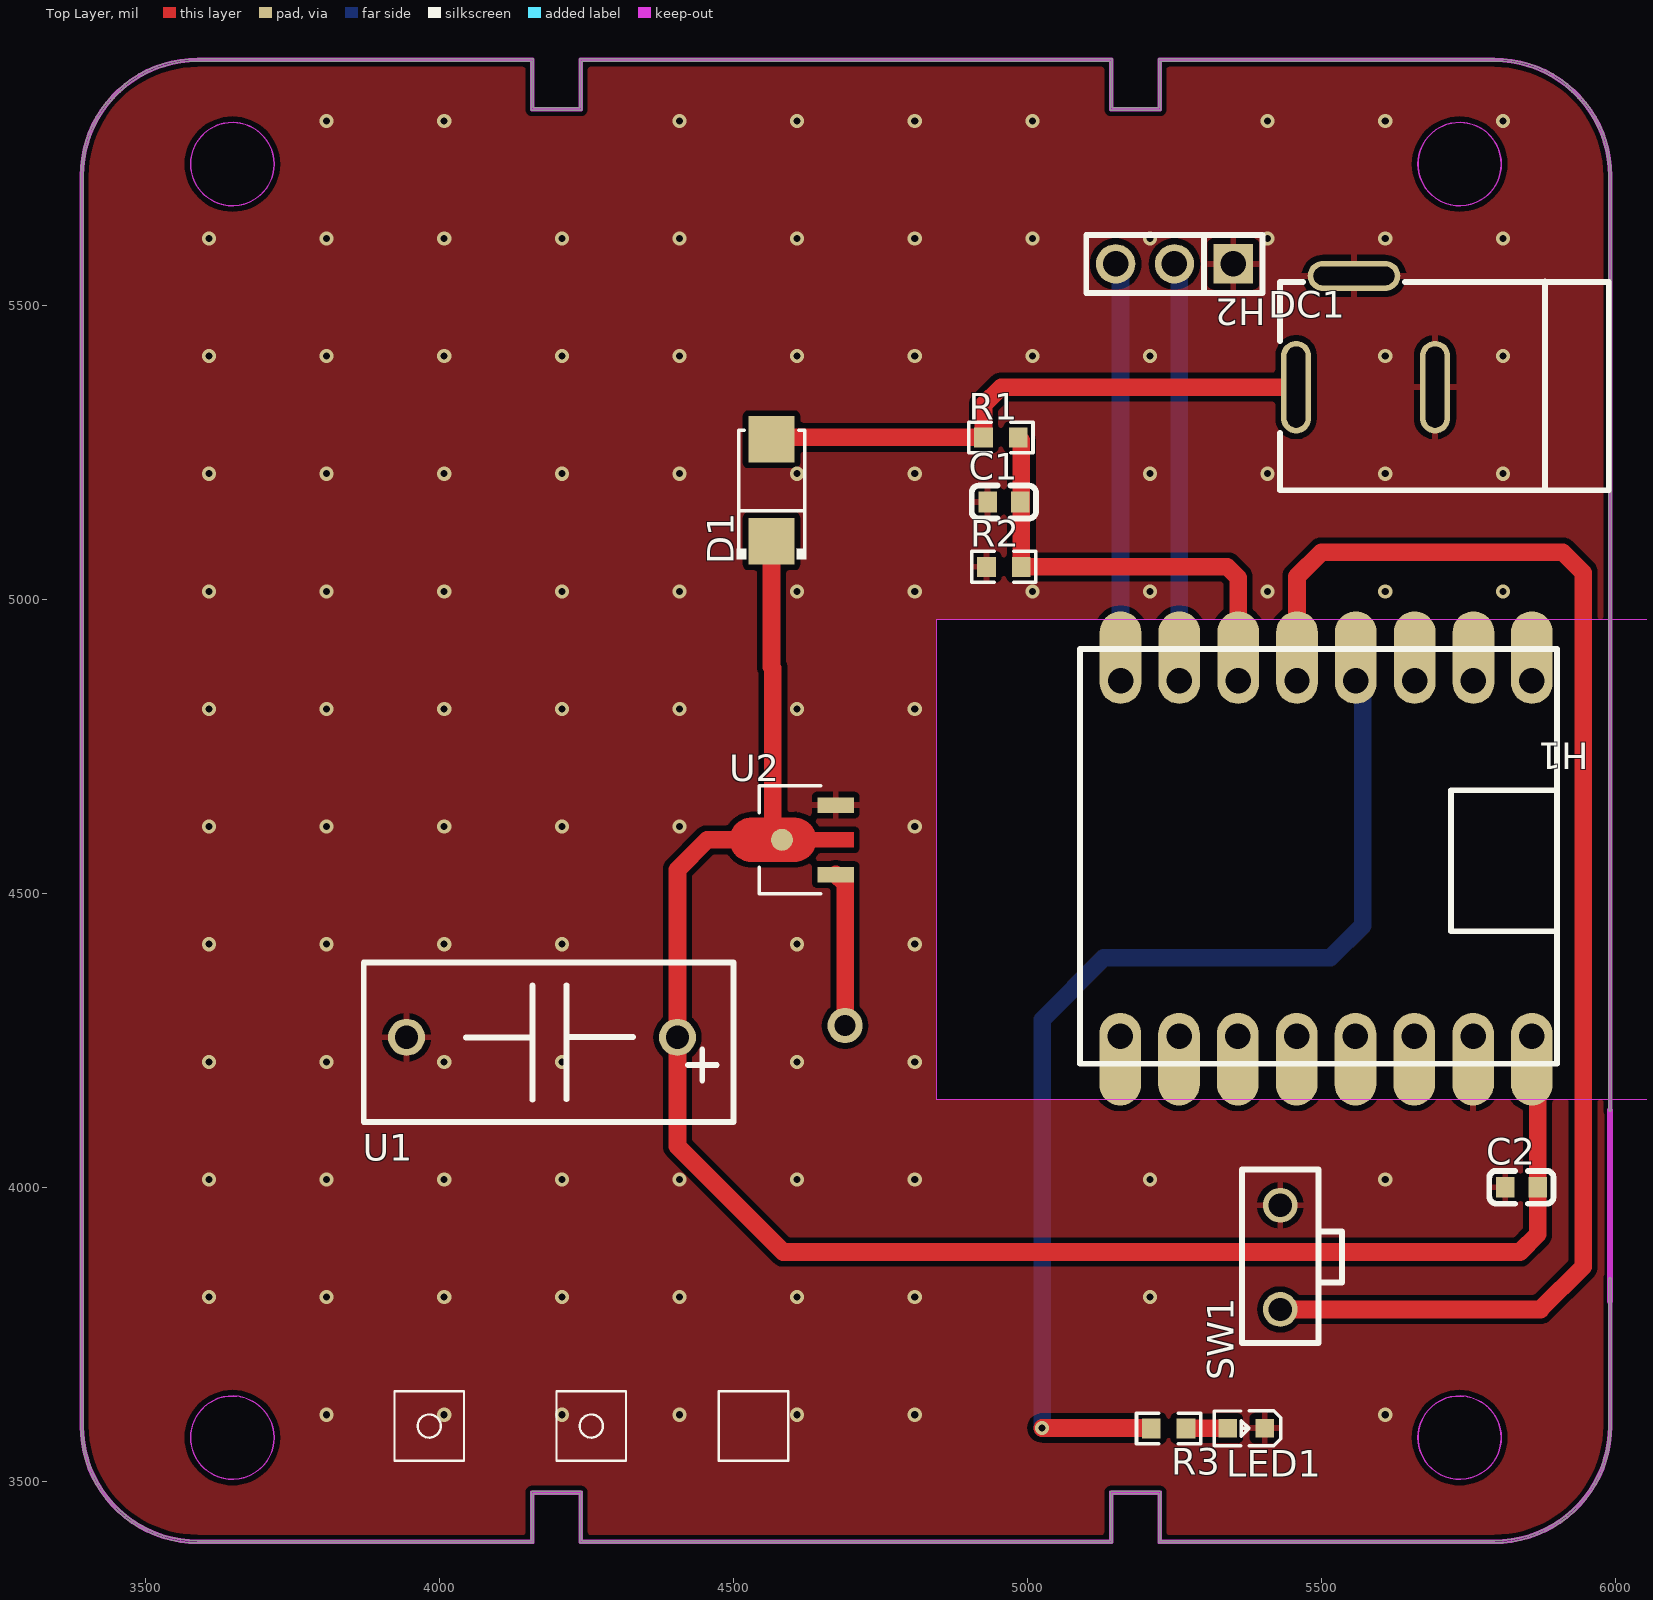
[diagram p0: Top Layer view]
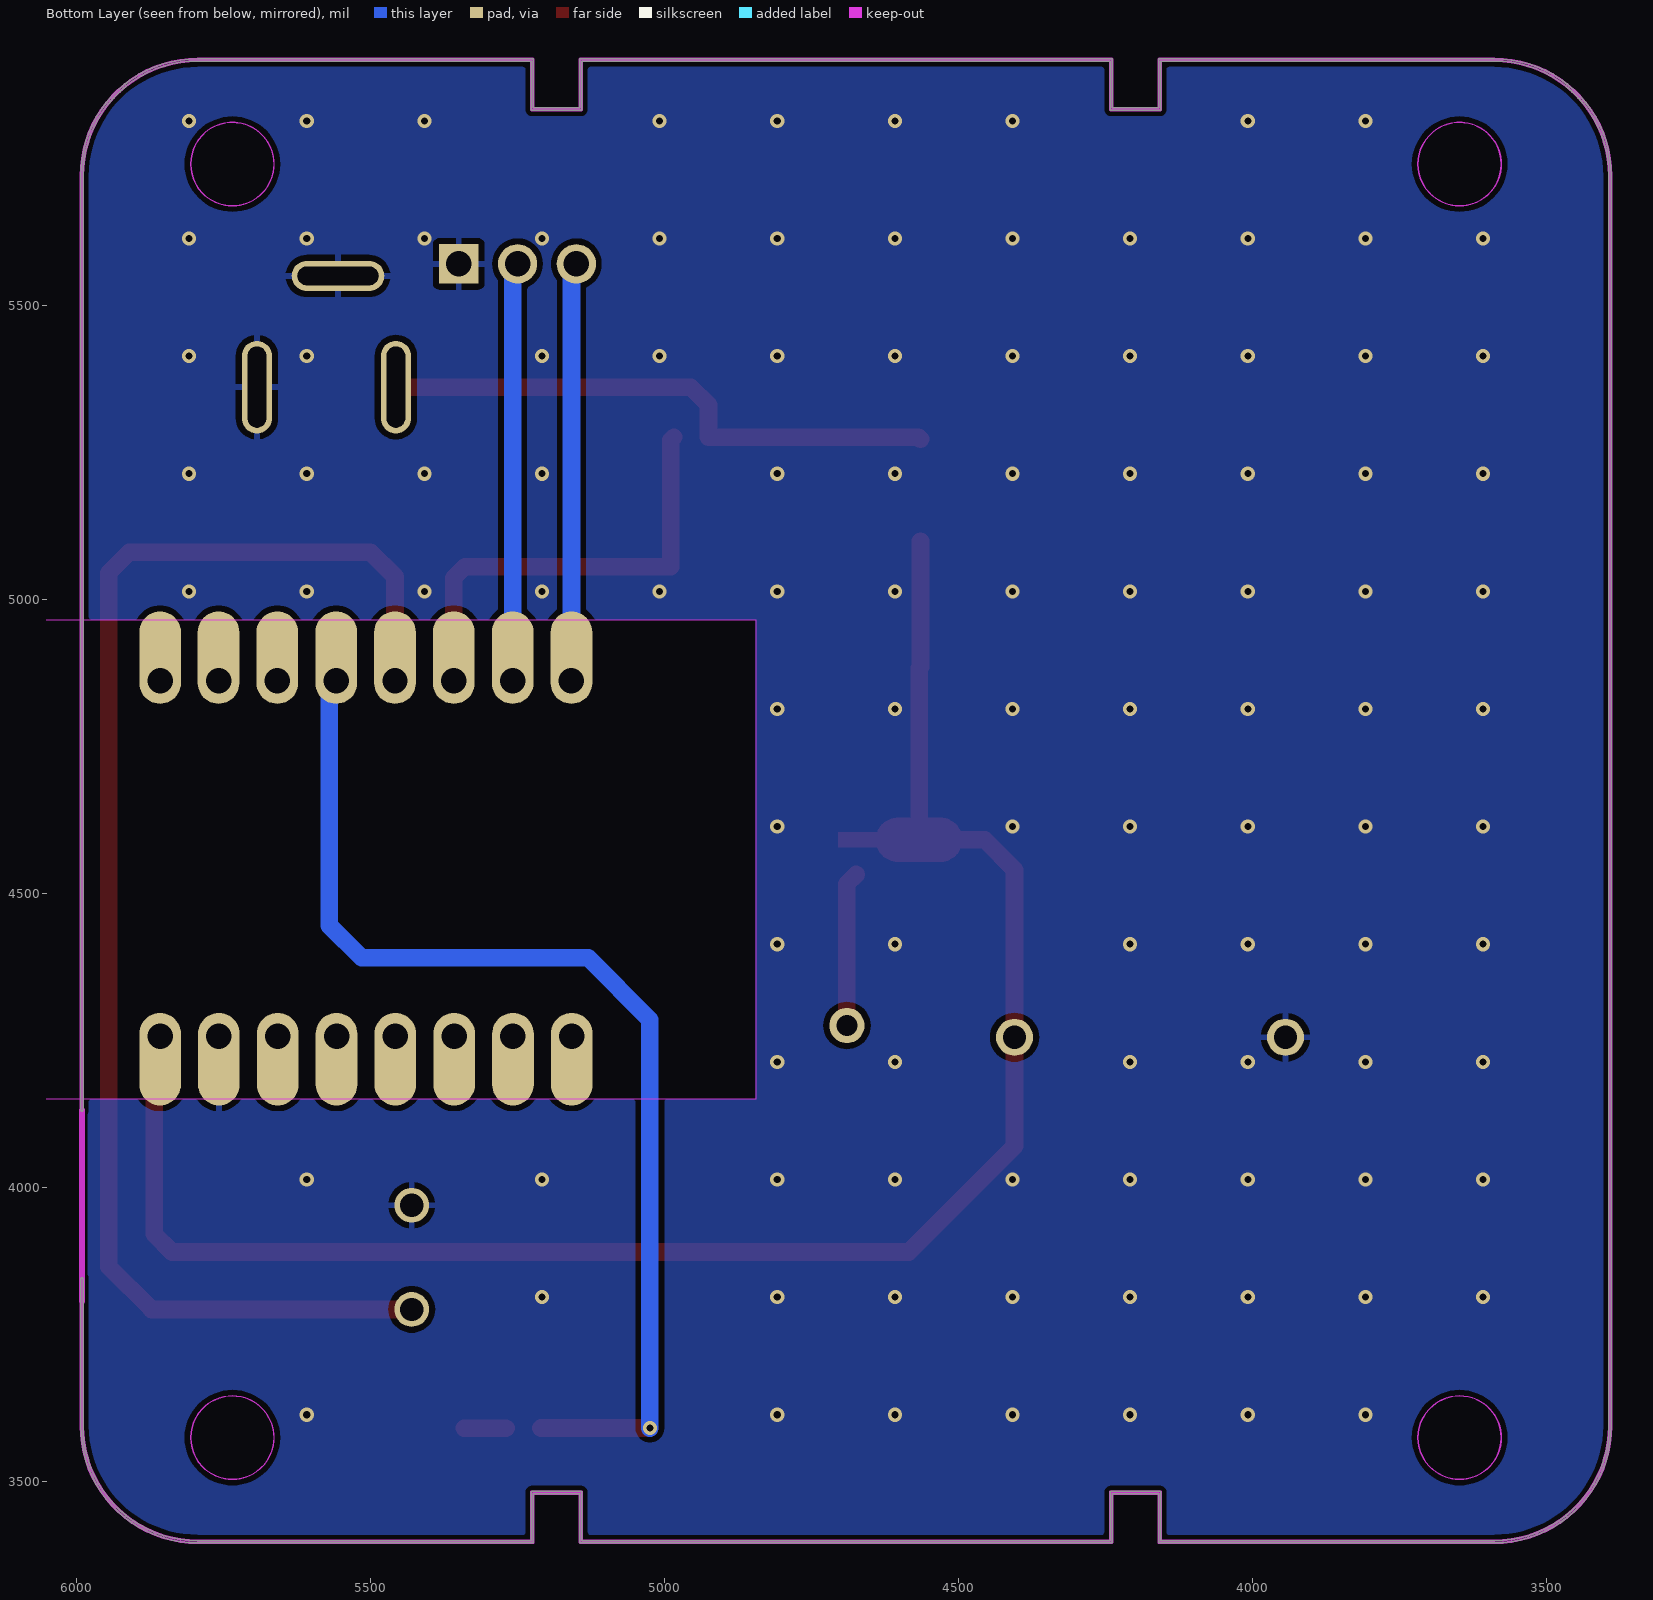
[diagram p1: Bottom Layer view, seen from below]
# Altium PCB MISC52083.pcbdoc
Units mil, origin at the board's own origin, x right, y up, seen from the top; angles counter-clockwise.
Board outline 2602.36 x 2523.62 mil, 2 copper layers (Top Layer, Bottom Layer), stack 62.206 mil thick; 13 components, 10 nets, 44 pads, 105 vias.

## Layer stack, top to bottom
Top Solder Mask Layer: solder mask 0.394, Dk 3.3
Top Layer: signal copper 1.379
Dielectric1: surface 59.449, FR4, Dk 4.5
Bottom Layer: signal copper 1.378
Bottom Solder Mask Layer: solder mask 0.394, Dk 3.3

## Board outline
5992.74,3594.03 cw(c5793.92,3594.03) 5793.92,3395.21 5224.89,3395.21 cw(c5224.89,3397.18) 5222.92,3397.18 5222.92,3478.94 5144.46,3478.94 5144.46,3397.18 cw(c5142.49,3397.18) 5142.49,3395.21 4240.63,3395.21 cw(c4240.63,3397.18) 4238.67,3397.18 4238.67,3478.94 4160.21,3478.94 4160.21,3397.18 cw(c4158.24,3397.18) 4158.24,3395.21 3589.2,3395.21 cw(c3589.2,3594.03) 3390.38,3594.03 3390.38,5720.02 cw(c3589.2,5720.02) 3589.2,5918.84 4158.24,5918.84 cw(c4158.24,5916.87) 4160.21,5916.87 4160.21,5835.12 4238.67,5835.12 4238.67,5916.87 cw(c4240.63,5916.87) 4240.63,5918.84 5142.49,5918.84 cw(c5142.49,5916.87) 5144.46,5916.87 5144.46,5835.12 5222.92,5835.12 5222.92,5916.87 cw(c5224.89,5916.87) 5224.89,5918.84 5793.92,5918.84 cw(c5793.92,5720.02) 5992.74,5720.02 5992.74,4131.27 cw(c5990.77,4131.27) 5990.77,4129.3 cw(c5990.77,4131.27) 5988.81,4131.27 5988.81,5720.02 ccw(c5793.92,5720.02) 5793.92,5914.9 5226.85,5914.9 5226.85,5833.16 cw(c5224.89,5833.16) 5224.89,5831.19 5142.49,5831.19 cw(c5142.49,5833.16) 5140.52,5833.16 5140.52,5914.9 4242.6,5914.9 4242.6,5833.16 cw(c4240.63,5833.16) 4240.63,5831.19 4158.24,5831.19 cw(c4158.24,5833.16) 4156.27,5833.16 4156.27,5914.9 3589.2,5914.9 ccw(c3589.2,5720.02) 3394.32,5720.02 3394.32,3594.03 ccw(c3589.2,3594.03) 3589.2,3399.15 4156.27,3399.15 4156.27,3480.91 cw(c4158.24,3480.91) 4158.24,3482.87 4240.63,3482.87 cw(c4240.63,3480.91) 4242.6,3480.91 4242.6,3399.15 5140.52,3399.15 5140.52,3480.91 cw(c5142.49,3480.91) 5142.49,3482.87 5224.89,3482.87 cw(c5224.89,3480.91) 5226.85,3480.91 5226.85,3399.15 5793.92,3399.15 ccw(c5793.92,3594.03) 5988.81,3594.03 5988.81,3844.2 cw(c5990.77,3844.2) 5990.77,3846.17 cw(c5990.77,3844.2) 5992.74,3844.2 5992.74,3594.03
cut-out: 3719.12,3574.35 cw(c3648.26,3574.35) 3577.39,3574.35 cw(c3648.26,3574.35)
cut-out: 5805.74,5739.7 cw(c5734.87,5739.7) 5664,5739.7 cw(c5734.87,5739.7)
cut-out: 3719.12,5739.7 cw(c3648.26,5739.7) 3577.39,5739.7 cw(c3648.26,5739.7)
cut-out: 5805.74,3574.35 cw(c5734.87,3574.35) 5664,3574.35 cw(c5734.87,3574.35)

## Design rules (kind name [scope] priority, off if disabled: settings)
BoardOutlineClearance copperThickness2oz_1 [All] p2 off: genericclearance=7.99 ignorepadtopadclearanceinfootprint=FALSE except(0: Arc-SplitContinuation Track-SplitContinuation SMDPad-SplitContinuation THPad-SplitContinuation Via-SplitContinuation Fill-SplitContinuation Region-SplitContinuation Poly-SplitContinuation Text-SplitContinuation Hole-SplitContinuation; 5.98: Arc-CutoutEdge SMDPad-CutoutEdge THPad-CutoutEdge Via-CutoutEdge Fill-CutoutEdge Region-CutoutEdge Text-CutoutEdge; 6.93: Hole-OutlineEdge Hole-CutoutEdge; 10: Poly-OutlineEdge Poly-CutoutEdge; 11.81: Arc-OutlineEdge Track-OutlineEdge SMDPad-OutlineEdge THPad-OutlineEdge Via-OutlineEdge Fill-OutlineEdge Region-OutlineEdge Text-OutlineEdge Track-CutoutEdge)
BoardOutlineClearance copperThickness1oz_1 [All] p4: genericclearance=4.02 ignorepadtopadclearanceinfootprint=FALSE except(0: Arc-SplitContinuation Track-SplitContinuation SMDPad-SplitContinuation THPad-SplitContinuation Via-SplitContinuation Fill-SplitContinuation Region-SplitContinuation Poly-SplitContinuation Text-SplitContinuation Hole-SplitContinuation; 6: SMDPad-CutoutEdge THPad-CutoutEdge Via-CutoutEdge Fill-CutoutEdge Region-CutoutEdge Text-CutoutEdge; 6.93: Hole-OutlineEdge Hole-CutoutEdge; 10: Poly-OutlineEdge Poly-CutoutEdge; 11.8: Arc-OutlineEdge Track-OutlineEdge SMDPad-OutlineEdge THPad-OutlineEdge Via-OutlineEdge Fill-OutlineEdge Region-OutlineEdge Text-OutlineEdge; 11.81: Arc-CutoutEdge Track-CutoutEdge)
Clearance copperThickness2oz [All] p1 off: gap=7.99 ignorepadtopadclearanceinfootprint=FALSE except(5.98: SMDPad-Track SMDPad-SMDPad THPad-Track SMDPad-THPad THPad-THPad Track-Via SMDPad-Via THPad-Via Via-Via Fill-Track Region-Track Fill-SMDPad Region-SMDPad Fill-THPad Region-THPad Fill-Via Region-Via Fill-Fill Fill-Region Region-Region Arc-Track Arc-SMDPad Arc-THPad Arc-Via Fill-Arc Region-Arc Arc-Arc Text-Track SMDPad-Text Text-THPad Text-Via Fill-Text Region-Text Arc-Text Text-Text; 6.93: Hole-Track Hole-SMDPad Hole-THPad Hole-Via Fill-Hole Region-Hole Hole-Arc Hole-Text; 10: Poly-Track Poly-SMDPad Poly-THPad Poly-Via Poly-Fill Poly-Region Poly-Poly Poly-Arc Poly-Text Poly-Hole)
Clearance copperThickness1oz [All] p3: gap=4.02 ignorepadtopadclearanceinfootprint=FALSE except(5.98: SMDPad-Track SMDPad-SMDPad THPad-Track SMDPad-THPad THPad-THPad Track-Via SMDPad-Via THPad-Via Via-Via Fill-Track Region-Track Fill-SMDPad Region-SMDPad Fill-THPad Region-THPad Fill-Via Region-Via Fill-Fill Fill-Region Region-Region; 6: Arc-Track Arc-SMDPad Arc-THPad Arc-Via Fill-Arc Region-Arc Arc-Arc Text-Track SMDPad-Text Text-THPad Text-Via Fill-Text Region-Text Arc-Text Text-Text; 6.93: Hole-Track Hole-SMDPad Hole-THPad Hole-Via Fill-Hole Region-Hole Hole-Arc Hole-Text; 10: Poly-Track Poly-SMDPad Poly-THPad Poly-Via Poly-Fill Poly-Region Poly-Poly Poly-Arc Poly-Text Poly-Hole)
Creepage creepage [All] p1: checkdistance=0 ignoreinternallayers=TRUE applytopolygonpour=TRUE
DiffPairsRouting differentialPair [All] p1: maxlimit=6 minlimit=6 mostfreqgap=6 toplayer_minwidth=5 toplayer_prefwidth=10 toplayer_maxwidth=100 toplayer_mingap=6 toplayer_prefgap=6 toplayer_maxgap=6 bottomlayer_minwidth=5 bottomlayer_prefwidth=10 bottomlayer_maxwidth=100 bottomlayer_mingap=6 bottomlayer_prefgap=6 bottomlayer_maxgap=6 maxuncoupledlength=10
HoleToHoleClearance otherClearance [All] p1: gap=11.81 allowstackedmicrovias=TRUE
Length netLength [All] p1: minlimit=0 maxlimit=0
MatchedLengths netLengthTolerance [All] p1: tolerance=1000
PasteMaskExpansion pasteMaskExpansion [All] p1: expansion=0
PlaneConnect innerPlane [All] p1: planeconnectstyle=Relief reliefexpansion=20 reliefentries=4 reliefconductorwidth=10 reliefairgap=10
PolygonConnect copperRegion [(InNet('GND'))] p1: connectstyle=Relief reliefconductorwidth=10 reliefentries=4 polygonreliefangle="90 Angle" airgapwidth=10 via.connectstyle=Relief via.reliefconductorwidth=10 via.reliefentries=4 via.polygonreliefangle="90 Angle" via.airgapwidth=10
RoutingVias viaSize [All] p1: holewidth=12.01 width=24.02 viastyle="Through Hole" minholewidth=11.81 minwidth=19.68 maxholewidth=248.03 maxwidth=393.7
SolderMaskExpansion solderMaskExpansion [IsVia] p1: expansion=-1000 istentingtop=TRUE
SolderMaskExpansion solderMaskExpansion [All] p2: expansion=2 istentingtop=FALSE
Width copperThickness2oz_2 [All] p1 off: maxlimit=100 minlimit=8 preferedwidth=10
Width copperThickness1oz_2 [All] p2: maxlimit=100 minlimit=5 preferedwidth=10

## Components (designator, comment, footprint, x,y, rotation, side; value= is the part's Value field where it differs from the comment)
C1 "100nF" C0603 4960,5165 r0 top
C2 "100nF" C0603 5840,4000 r0 top
D1 "SS34" SMA_L4.3-W2.6-LS5.2-RD 4565,5185 r90 top
DC1 "" DC-2.0 5580,5350 r0 top
H1 "" HDR-TH_16P-P2.54-V-F-R2-C8-S2.54-1 5545,4865 r180 top
H2 "" HDR-TH_3P-P2.54-V-M 5250,5570 r180 top
LED1 "" LED_0603 5370,3590 r180 top
R1 "10K" R0603 4955,5275 r180 top
R2 "15K" R0603 4960,5055 r0 top
R3 "1K" R0603 5240,3590 r0 top
SW1 "" Key_TH_3.5x6x4.3 5430,3835 r90 top
U1 "2F" CAP-TH_BD8.0-P3.50-D0.6-FD_GDC02R7R205LD0816 4405,4255 r180 top
U2 "HT7033A-1" SOT-89-3_L4.5-W2.5-P1.50-LS4.2-BR 4620.69,4590.78 r0 top

## Footprints (in the part's own frame and the unit in brackets; to place one, negate y for a bottom-side part, rotate by r counter-clockwise, add the part's x,y. Pads: shape width x height; smd on the part's side, far side on the other; paste and mask are expansions set on the pad)
C0603 [mm]
  rect 0.8x0.9 smd: 1(-0.7,0) 2(0.7,0)
  silkscreen extent -1.39,-0.71 1.39,0.71
CAP-TH_BD8.0-P3.50-D0.6-FD_GDC02R7R205LD0816 [mm]
  round 1.6 hole 1: 1(0,0) 2(11.7,0)
  silkscreen extent -2.42,-3.22 13.55,3.65
DC-2.0 [mil]
  oval 157.5x51.2 hole 31.5 slot 137.8 at 0 deg paste+0 mask+2: 2(-24.7,199.5)
  oval 51.2x157.5 hole 31.5 slot 137.8 at 90 deg paste+0 mask+2: 3(113.1,10.5) 4(-123.1,10.5)
  silkscreen extent -151,-165 408,190
HDR-TH_3P-P2.54-V-M [mm]
  rect 1.7x1.7 hole 1.1: 1(-2.54,0)
  round 1.7 hole 1.1: 2(0,0) 3(2.54,0)
  silkscreen extent -3.81,-1.25 3.81,1.25
HDR-TH_16P-P2.54-V-F-R2-C8-S2.54-1 [mm]
  oval 1.8x4 hole 1.1 copper offset 0,1: 1(-7.945,15.439) 3(-5.405,15.439) 5(-2.865,15.439) 7(-0.325,15.439) 9(2.215,15.439) 11(4.755,15.439) 13(7.295,15.439) 15(9.835,15.439)
  oval 1.8x4 hole 1.1 copper offset 0,-1: 2(-7.945,0.096) 4(-5.42,0.096) 6(-2.88,0.096) 8(-0.34,0.096) 10(2.2,0.096) 12(4.74,0.096) 14(7.28,0.096) 16(9.82,0.096)
  silkscreen extent -9.03,-1.27 11.57,16.64
Key_TH_3.5x6x4.3 [mm]
  round 1.5 hole 1 paste+0 mask+0.051: A(-1.085,0) B(3.415,0)
  silkscreen extent -2.54,-2.67 4.95,1.65
LED_0603 [mil]
  rect 31.5x31.5 smd paste+0 mask+2: 1(-33.5,-0.4) 2(29.5,-0.2)
  silkscreen extent -61,-30 53,30
R0603 [mil]
  rect 31.75x34.02 smd paste-3937.01 mask+2: 1(-29.66,0) 2(29.66,0)
  silkscreen extent -55,-26 55,26
SMA_L4.3-W2.6-LS5.2-RD [mm]
  rect 2x2 smd: 1(-2.2,0) 2(2.2,0)
  silkscreen extent -2.98,-1.5 2.6,1.5
SOT-89-3_L4.5-W2.5-P1.50-LS4.2-BR [mm]
  rect 1.575x0.672 smd: 1(1.356,-1.5) 3(1.356,1.5)
  round 0.95 smd: 2(-0.966,0)
  Top Layer region: -2.283,0.95 -0.429,0.95 -0.384,0.949 -0.34,0.946 -0.296,0.94 -0.252,0.933 -0.208,0.924 -0.165,0.912 -0.123,0.899 -0.081,0.884 -0.04,0.866 0,0.847 0.04,0.826 0.078,0.803 0.115,0.779 0.151,0.752 0.185,0.724 0.219,0.695 0.251,0.664 0.281,0.631 0.31,0.597 0.337,0.562 0.362,0.525 0.386,0.488 0.408,0.449 0.428,0.409 0.447,0.33 2.144,0.33 2.144,-0.33 0.447,-0.33 0.428,-0.409 0.408,-0.449 0.386,-0.488 0.362,-0.526 0.337,-0.562 0.31,-0.597 0.281,-0.631 0.251,-0.664 0.219,-0.695 0.185,-0.725 0.151,-0.753 0.115,-0.779 0.078,-0.804 0.04,-0.827 0,-0.848 -0.04,-0.867 -0.081,-0.884 -0.123,-0.899 -0.165,-0.913 -0.208,-0.924 -0.252,-0.934 -0.296,-0.941 -0.34,-0.946 -0.384,-0.949 -0.429,-0.95 -2.283,-0.95 -2.328,-0.949 -2.372,-0.946 -2.416,-0.941 -2.46,-0.934 -2.504,-0.924 -2.547,-0.913 -2.589,-0.899 -2.631,-0.884 -2.672,-0.867 -2.713,-0.848 -2.752,-0.827 -2.79,-0.804 -2.827,-0.779 -2.863,-0.753 -2.898,-0.725 -2.931,-0.695 -2.963,-0.664 -2.993,-0.631 -3.022,-0.597 -3.049,-0.562 -3.075,-0.526 -3.098,-0.488 -3.12,-0.449 -3.141,-0.409 -3.159,-0.369 -3.175,-0.327 -3.189,-0.285 -3.202,-0.242 -3.212,-0.199 -3.22,-0.155 -3.227,-0.111 -3.231,-0.067 -3.233,-0.022 -3.233,0.022 -3.231,0.067 -3.227,0.111 -3.22,0.155 -3.212,0.199 -3.202,0.242 -3.189,0.285 -3.175,0.327 -3.159,0.369 -3.141,0.409 -3.12,0.449 -3.098,0.488 -3.075,0.525 -3.049,0.562 -3.022,0.597 -2.993,0.631 -2.963,0.664 -2.931,0.695 -2.898,0.724 -2.863,0.752 -2.827,0.779 -2.79,0.803 -2.752,0.826 -2.713,0.847 -2.672,0.866 -2.631,0.884 -2.589,0.899 -2.547,0.912 -2.504,0.924 -2.46,0.933 -2.416,0.94 -2.372,0.946 -2.328,0.949
  silkscreen extent -1.95,-2.33 0.7,2.33

## Free pads (board coordinates)
  round 60 hole 36: 1(4690,4275)

## Via types
v1: diameter 24.02, hole 12, Top Layer to Bottom Layer, 105 vias

## Nets (pads, with @x,y where several pads share a name; then routed paths per layer and width w, separated by ;. In a path a pad name is that pad's centre, name@x,y a point inside that pad or via, vN(x,y) a via of type N, cw(c..) or ccw(c..) an arc to the next point about the centre after c; other vN are vias at no path point)
5V: C2.2 D1.1 H1.1 U1.1 U2.2 | length 3013.3
  Top Layer w30: D1.1 4565,4885 4567.3,4882.7 4567.3,4590.78 4455.78,4590.78 4405,4540 U1.1 4405,4070 4585,3890 5837.56,3890 5867.56,3920 C2.2 5867.56,4208.03 H1.1@5857.8,4217.8
$1N4: C1.2 H1.12 R1.1 R2.2 | length 734.4
  Top Layer w30: R1.1 4989.66,5270 R2.2 5340,5055 5358.39,5036.61 H1.12@5358.39,4900.59
$1N5: H1.8 R3.1 | length 1951.6
  Top Layer w30: v1(5025,3590.78) 5209.56,3590.78 R3.1
  Bottom Layer w30: v1(5025,3590.78) 5025,4285 5130,4390 5515,4390 5570,4445 5570,4888.98 H1.8@5558.39,4900.59
$1N10: H1.16 H2.3 | length 672.9
  Bottom Layer w30: H2.3 5158.39,5561.61 H1.16@5158.39,4900.59
$1N11: H1.14 H2.2 | length 672.9
  Bottom Layer w30: H2.2 5258.39,5561.61 H1.14@5258.39,4900.59
$1N13: H1.10 SW1.A | length 2381.3
  Top Layer w30: SW1.A 5872.29,3792.29 5945,3865 5945,5045 5910,5080 5500,5080 5458.39,5038.39 H1.10@5458.39,4900.59
$1N15: LED1.2 R3.2 | length 70.9
  Top Layer w30: R3.2 5340.3,3590 LED1.2
+5V: D1.2 DC1.4 R1.2 | length 961.1
  Top Layer w30: D1.2 4568.39,5275 R1.2 4925.34,5330.34 4955.5,5360.5 DC1.4
GND: C1.1 C2.1 DC1.2 DC1.3 H1.3 H2.1 LED1.1 R2.1 SW1.B U1.2 U2.3
  other v1: 3808.42,3613.25 4008.42,3613.25 4208.42,3613.25 4408.42,3613.25 4608.42,3613.25 4808.42,3613.25 5608.42,3613.25 3608.42,3813.25 3808.42,3813.25 4008.42,3813.25 4208.42,3813.25 4408.42,3813.25 4608.42,3813.25 4808.42,3813.25 5208.42,3813.25 3608.42,4013.25 3808.42,4013.25 4008.42,4013.25 4208.42,4013.25 4408.42,4013.25 4608.42,4013.25 4808.42,4013.25 5208.42,4013.25 5608.42,4013.25 3608.42,4213.25 3808.42,4213.25 4008.42,4213.25 4208.42,4213.25 4608.42,4213.25 4808.42,4213.25 3608.42,4413.25 3808.42,4413.25 4008.42,4413.25 4208.42,4413.25 4608.42,4413.25 4808.42,4413.25 3608.42,4613.25 3808.42,4613.25 4008.42,4613.25 4208.42,4613.25 4408.42,4613.25 4808.42,4613.25 3608.42,4813.25 3808.42,4813.25 4008.42,4813.25 4208.42,4813.25 4408.42,4813.25 4608.42,4813.25 4808.42,4813.25 3608.42,5013.25 3808.42,5013.25 4008.42,5013.25 4208.42,5013.25 4408.42,5013.25 4608.42,5013.25 4808.42,5013.25 5008.42,5013.25 5208.42,5013.25 5408.42,5013.25 5608.42,5013.25 5808.42,5013.25 3608.42,5213.25 3808.42,5213.25 4008.42,5213.25 4208.42,5213.25 4408.42,5213.25 4608.42,5213.25 4808.42,5213.25 5208.42,5213.25 5408.42,5213.25 5608.42,5213.25 5808.42,5213.25 3608.42,5413.25 3808.42,5413.25 4008.42,5413.25 4208.42,5413.25 4408.42,5413.25 4608.42,5413.25 4808.42,5413.25 5008.42,5413.25 5208.42,5413.25 5608.42,5413.25 5808.42,5413.25 3608.42,5613.25 3808.42,5613.25 4008.42,5613.25 4208.42,5613.25 4408.42,5613.25 4608.42,5613.25 4808.42,5613.25 5008.42,5613.25 5208.42,5613.25 5408.42,5613.25 5608.42,5613.25 5808.42,5613.25 3808.42,5813.25 4008.42,5813.25 4408.42,5813.25 4608.42,5813.25 4808.42,5813.25 5008.42,5813.25 5408.42,5813.25 5608.42,5813.25 5808.42,5813.25
RST: pad.1 U2.1 | length 263.3
  Top Layer w30: U2.1 4690,4515.82 pad.1
pads on no net: H1.2 H1.4 H1.5 H1.6 H1.7 H1.9 H1.11 H1.13 H1.15

## Polygon pours and split planes (outlines as drawn)
GND on Top Layer (solid, remove dead copper, pour order 0): 3000,6080 3000,3000 6340,3000 6340,6080
GND on Bottom Layer (solid, remove dead copper, pour order 2): 3130,6120 3130,3010 6415,3010 6415,6120

## Keep-outs
Board Outline Layer:
  region: 3719.12,3574.35 cw(c3648.26,3574.35) 3577.39,3574.35 cw(c3648.26,3574.35)
  circle w0.1: c3648.26,3574.35 r70.87
  region: 3719.12,3574.35 3718.73,3566.94 3717.57,3559.61 3715.65,3552.45 3712.99,3545.52 3709.63,3538.91 3705.59,3532.69 3700.92,3526.93 3695.67,3521.68 3689.91,3517.02 3683.69,3512.98 3677.08,3509.61 3670.15,3506.95 3662.99,3505.03 3655.66,3503.87 3648.26,3503.48 3640.85,3503.87 3633.52,3505.03 3626.36,3506.95 3619.43,3509.61 3612.82,3512.98 3606.6,3517.02 3600.84,3521.68 3595.59,3526.93 3590.92,3532.69 3586.88,3538.91 3583.52,3545.52 3580.86,3552.45 3578.94,3559.61 3577.78,3566.94 3577.39,3574.35 3577.78,3581.76 3578.94,3589.08 3580.86,3596.25 3583.52,3603.17 3586.88,3609.78 3590.92,3616 3595.59,3621.77 3600.84,3627.01 3606.6,3631.68 3612.82,3635.72 3619.43,3639.09 3626.36,3641.75 3633.52,3643.67 3640.85,3644.83 3648.26,3645.21 3655.66,3644.83 3662.99,3643.67 3670.15,3641.75 3677.08,3639.09 3683.69,3635.72 3689.91,3631.68 3695.67,3627.01 3700.92,3621.77 3705.59,3616 3709.63,3609.78 3712.99,3603.17 3715.65,3596.25 3717.57,3589.08 3718.73,3581.76
  region: 5805.74,5739.7 cw(c5734.87,5739.7) 5664,5739.7 cw(c5734.87,5739.7)
  circle w0.1: c5734.87,5739.7 r70.87
  region: 5805.74,5739.7 5805.35,5732.29 5804.19,5724.97 5802.27,5717.8 5799.61,5710.88 5796.24,5704.27 5792.2,5698.05 5787.53,5692.28 5782.29,5687.04 5776.52,5682.37 5770.3,5678.33 5763.69,5674.96 5756.77,5672.3 5749.6,5670.38 5742.28,5669.22 5734.87,5668.84 5727.46,5669.22 5720.14,5670.38 5712.97,5672.3 5706.05,5674.96 5699.44,5678.33 5693.22,5682.37 5687.45,5687.04 5682.21,5692.28 5677.54,5698.05 5673.5,5704.27 5670.13,5710.88 5667.47,5717.8 5665.55,5724.97 5664.39,5732.29 5664,5739.7 5664.39,5747.11 5665.55,5754.44 5667.47,5761.6 5670.13,5768.53 5673.5,5775.14 5677.54,5781.36 5682.21,5787.12 5687.45,5792.37 5693.22,5797.03 5699.44,5801.07 5706.05,5804.44 5712.97,5807.1 5720.14,5809.02 5727.46,5810.18 5734.87,5810.57 5742.28,5810.18 5749.6,5809.02 5756.77,5807.1 5763.69,5804.44 5770.3,5801.07 5776.52,5797.03 5782.29,5792.37 5787.53,5787.12 5792.2,5781.36 5796.24,5775.14 5799.61,5768.53 5802.27,5761.6 5804.19,5754.44 5805.35,5747.11
  region: 3719.12,5739.7 cw(c3648.26,5739.7) 3577.39,5739.7 cw(c3648.26,5739.7)
  circle w0.1: c3648.26,5739.7 r70.87
  region: 3719.12,5739.7 3718.73,5732.29 3717.57,5724.97 3715.65,5717.8 3712.99,5710.88 3709.63,5704.27 3705.59,5698.05 3700.92,5692.28 3695.67,5687.04 3689.91,5682.37 3683.69,5678.33 3677.08,5674.96 3670.15,5672.3 3662.99,5670.38 3655.66,5669.22 3648.26,5668.84 3640.85,5669.22 3633.52,5670.38 3626.36,5672.3 3619.43,5674.96 3612.82,5678.33 3606.6,5682.37 3600.84,5687.04 3595.59,5692.28 3590.92,5698.05 3586.88,5704.27 3583.52,5710.88 3580.86,5717.8 3578.94,5724.97 3577.78,5732.29 3577.39,5739.7 3577.78,5747.11 3578.94,5754.44 3580.86,5761.6 3583.52,5768.53 3586.88,5775.14 3590.92,5781.36 3595.59,5787.12 3600.84,5792.37 3606.6,5797.03 3612.82,5801.07 3619.43,5804.44 3626.36,5807.1 3633.52,5809.02 3640.85,5810.18 3648.26,5810.57 3655.66,5810.18 3662.99,5809.02 3670.15,5807.1 3677.08,5804.44 3683.69,5801.07 3689.91,5797.03 3695.67,5792.37 3700.92,5787.12 3705.59,5781.36 3709.63,5775.14 3712.99,5768.53 3715.65,5761.6 3717.57,5754.44 3718.73,5747.11
  region: 5805.74,3574.35 cw(c5734.87,3574.35) 5664,3574.35 cw(c5734.87,3574.35)
  circle w0.1: c5734.87,3574.35 r70.87
  region: 5805.74,3574.35 5805.35,3566.94 5804.19,3559.61 5802.27,3552.45 5799.61,3545.52 5796.24,3538.91 5792.2,3532.69 5787.53,3526.93 5782.29,3521.68 5776.52,3517.02 5770.3,3512.98 5763.69,3509.61 5756.77,3506.95 5749.6,3505.03 5742.28,3503.87 5734.87,3503.48 5727.46,3503.87 5720.14,3505.03 5712.97,3506.95 5706.05,3509.61 5699.44,3512.98 5693.22,3517.02 5687.45,3521.68 5682.21,3526.93 5677.54,3532.69 5673.5,3538.91 5670.13,3545.52 5667.47,3552.45 5665.55,3559.61 5664.39,3566.94 5664,3574.35 5664.39,3581.76 5665.55,3589.08 5667.47,3596.25 5670.13,3603.17 5673.5,3609.78 5677.54,3616 5682.21,3621.77 5687.45,3627.01 5693.22,3631.68 5699.44,3635.72 5706.05,3639.09 5712.97,3641.75 5720.14,3643.67 5727.46,3644.83 5734.87,3645.21 5742.28,3644.83 5749.6,3643.67 5756.77,3641.75 5763.69,3639.09 5770.3,3635.72 5776.52,3631.68 5782.29,3627.01 5787.53,3621.77 5792.2,3616 5796.24,3609.78 5799.61,3603.17 5802.27,3596.25 5804.19,3589.08 5805.35,3581.76
  region: 4845,4965 4845,4150 6110,4150 6110,4965
  lines w3.94: 3390.38,3594.03 ccw(c3589.2,3594.03) 3589.2,3395.21 4158.24,3395.21 ccw(c4158.24,3397.18) 4160.21,3397.18 4160.21,3478.94 4238.67,3478.94 4238.67,3397.18 ccw(c4240.63,3397.18) 4240.63,3395.21 5142.49,3395.21 ccw(c5142.49,3397.18) 5144.46,3397.18 5144.46,3478.94 5222.92,3478.94 5222.92,3397.18 ccw(c5224.89,3397.18) 5224.89,3395.21 5793.92,3395.21 ccw(c5793.92,3594.03) 5992.74,3594.03 5992.74,3844.2 ccw(c5990.77,3844.2) 5990.77,3846.17 ccw(c5990.77,3844.2) 5988.81,3844.2 5988.81,3594.03 cw(c5793.92,3594.03) 5793.92,3399.15 5226.85,3399.15 5226.85,3480.91 ccw(c5224.89,3480.91) 5224.89,3482.87 5142.49,3482.87 ccw(c5142.49,3480.91) 5140.52,3480.91 5140.52,3399.15 4242.6,3399.15 4242.6,3480.91 ccw(c4240.63,3480.91) 4240.63,3482.87 4158.24,3482.87 ccw(c4158.24,3480.91) 4156.27,3480.91 4156.27,3399.15 3589.2,3399.15 cw(c3589.2,3594.03) 3394.32,3594.03 3394.32,5720.02 cw(c3589.2,5720.02) 3589.2,5914.9 4156.27,5914.9 4156.27,5833.16 ccw(c4158.24,5833.16) 4158.24,5831.19 4240.63,5831.19 ccw(c4240.63,5833.16) 4242.6,5833.16 4242.6,5914.9 5140.52,5914.9 5140.52,5833.16 ccw(c5142.49,5833.16) 5142.49,5831.19 5224.89,5831.19 ccw(c5224.89,5833.16) 5226.85,5833.16 5226.85,5914.9 5793.92,5914.9 cw(c5793.92,5720.02) 5988.81,5720.02 5988.81,4131.27 ccw(c5990.77,4131.27) 5990.77,4129.3 ccw(c5990.77,4131.27) 5992.74,4131.27 5992.74,5720.02 ccw(c5793.92,5720.02) 5793.92,5918.84 5224.89,5918.84 ccw(c5224.89,5916.87) 5222.92,5916.87 5222.92,5835.12 5144.46,5835.12 5144.46,5916.87 ccw(c5142.49,5916.87) 5142.49,5918.84 4240.63,5918.84 ccw(c4240.63,5916.87) 4238.67,5916.87 4238.67,5835.12 4160.21,5835.12 4160.21,5916.87 ccw(c4158.24,5916.87) 4158.24,5918.84 3589.2,5918.84 ccw(c3589.2,5720.02) 3390.38,5720.02 3390.38,3594.03
  lines w10: 5990.77,3805.53 5990.77,4131.27

## Silkscreen, mask and mechanical layers (free items; w line width, h text height)
Top Silkscreen Layer:
  circle w3.94: c3982.9,3594.03 r19.68
  circle w3.94: c4258.49,3594.03 r19.68
  lines w3.94: 3923.85,3534.98 4041.96,3534.98 4041.96,3653.09 3923.85,3653.09 3923.85,3534.98 ; 4199.44,3534.98 4199.44,3653.09 4317.55,3653.09 4317.55,3534.98 4199.44,3534.98 ; 4475.03,3534.98 4475.03,3653.09 4593.14,3653.09 4593.14,3534.98 4475.03,3534.98
Mechanical Layer:
  circle w0.1: c3648.26,3574.35 r70.87
  circle w0.1: c5734.87,5739.7 r70.87
  circle w0.1: c3648.26,5739.7 r70.87
  circle w0.1: c5734.87,3574.35 r70.87

## Dimensions
5992.74,4362.75 to 5860,4362.75 on Document Layer